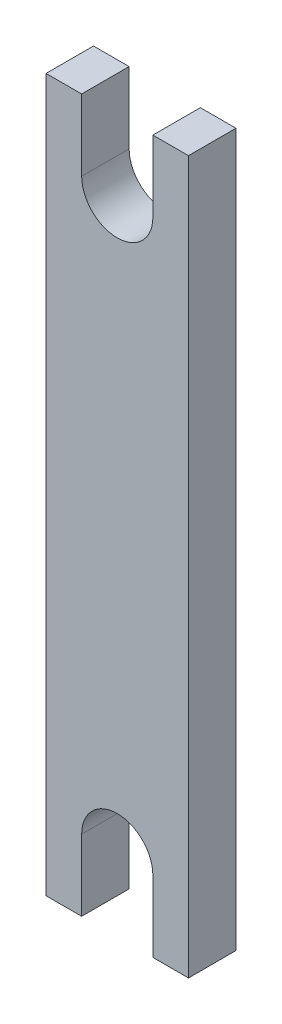
SolidWorks part; units mm, degrees
ref_plane "Front Plane" through (0, 0, 0) normal (0, 0, 1) x (1, 0, 0)
ref_plane "Top Plane" through (0, 0, 0) normal (0, 1, 0) x (1, 0, 0)
ref_plane "Right Plane" through (0, 0, 0) normal (1, 0, 0) x (0, 0, -1)
sketch "Sketch1" plane through (0, 0, 0) normal (0, 0, 1) x (1, 0, 0)
  line L0 (3, 15) -> (3, -15)
  line L1 (3, -15) -> (1.5, -15)
  line L2 (-1.5, -15) -> (-1.5, -12)
  line L3 (3, 15) -> (1.5, 15)
  line L4 (-1.5, 15) -> (-1.5, 12)
  line L5 (0, 9.8986) -> (0, -8.339) construction
  line L6 (-3, -15) -> (-1.5, -15)
  line L7 (1.5, -15) -> (1.5, -12)
  line L8 (1.5, 15) -> (1.5, 12)
  line L9 (-3, 15) -> (-1.5, 15)
  line L10 (-3, 15) -> (-3, -15)
  arc A0 (-1.5, 12) -> (1.5, 12) centre (0, 12) ccw
  arc A1 (1.5, -12) -> (-1.5, -12) centre (0, -12) ccw
  dimension "D1" = 1.5
  dimension "D2" = 1.5
  dimension "D3" = 6
  dimension "D4" = 3
  dimension "D5" = 30
  dimension "D6" = 3
  dimension "D7" = 15
extrude "Boss-Extrude1" add sketch "Sketch1" along normal blind 2
